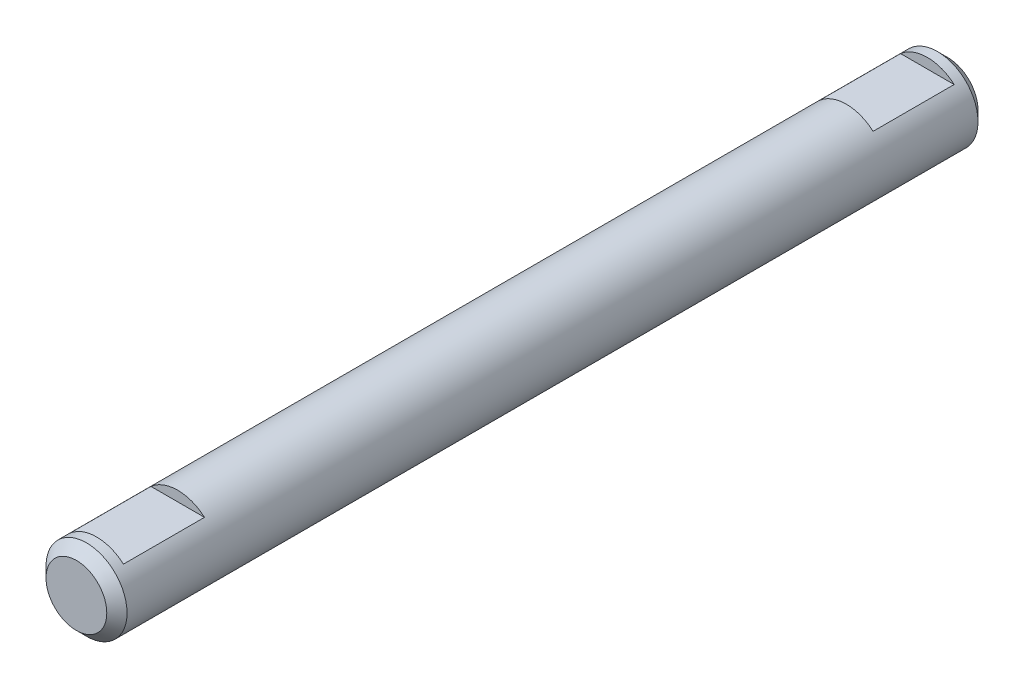
SolidWorks part; units mm, degrees
ref_plane "Front Plane" through (0, 0, 0) normal (0, 0, 1) x (1, 0, 0)
ref_plane "Top Plane" through (0, 0, 0) normal (0, 1, 0) x (1, 0, 0)
ref_plane "Right Plane" through (0, 0, 0) normal (1, 0, 0) x (0, 0, -1)
sketch "Sketch1" plane through (0, 0, 0) normal (0, 0, 1) x (1, 0, 0)
  circle A0 centre (0, 0) radius 2
  dimension "D1" = 4
extrude "Boss-Extrude1" add sketch "Sketch1" along normal mid plane 43
ref_plane "Plane1" through (0, 2, 0) normal (0, 1, 0) x (-1, 0, 0)
sketch "Sketch2" plane through (0, 2, 0) normal (0, 1, 0) x (-1, 0, 0)
  line L0 (-2, -21.5) -> (2, -21.5) construction
  line L1 (-7.7093, 20.5) -> (7.7093, 20.5)
  line L2 (-7.7093, 20.5) -> (-7.7093, 16.5)
  line L3 (-7.7093, 16.5) -> (7.7093, 16.5)
  line L4 (7.7093, 20.5) -> (7.7093, 16.5)
  line L5 (-5.0318, -16.5) -> (6.786, -16.5)
  line L6 (-5.0318, -16.5) -> (-5.0318, -20.5)
  line L7 (-5.0318, -20.5) -> (6.786, -20.5)
  line L8 (6.786, -16.5) -> (6.786, -20.5)
  line L9 (2, 21.5) -> (-2, 21.5) construction
  dimension "D1" = 4
  dimension "D2" = 4
  dimension "D3" = 1
  dimension "D4" = 1
extrude "Cut-Extrude1" cut sketch "Sketch2" against normal blind 0.5
chamfer "Chamfer1" distance 0.5 angle 45 2 edges at (2, 0, 21.5) (2, 0, -21.5)
